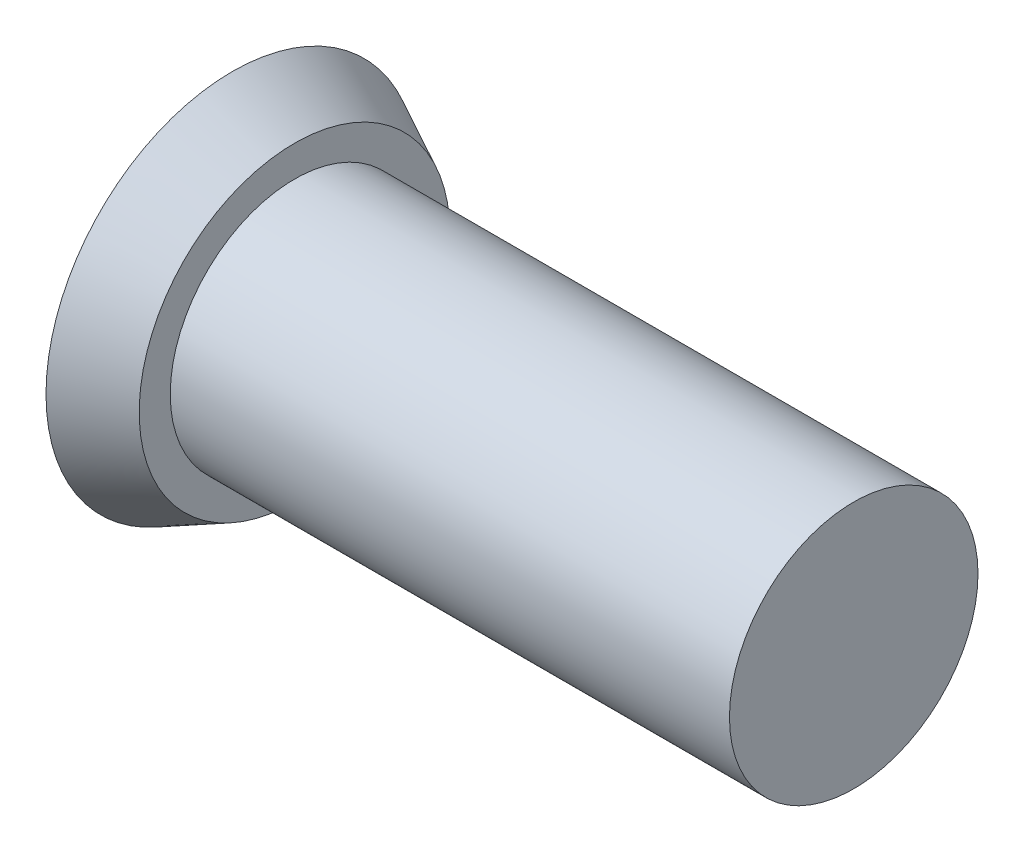
SolidWorks part; units mm, degrees
ref_plane "Front Plane" through (0, 0, 0) normal (0, 0, 1) x (1, 0, 0)
ref_plane "Top Plane" through (0, 0, 0) normal (0, 1, 0) x (1, 0, 0)
ref_plane "Right Plane" through (0, 0, 0) normal (1, 0, 0) x (0, 0, -1)
other "Configuration Table"
sketch "Sketch1" plane through (0, 0, 0) normal (0, 0, 1) x (1, 0, 0)
  line L0 (0, 0) -> (0, 3)
  line L1 (0, 3) -> (1, 2.5)
  line L2 (1, 2.5) -> (1, 2)
  line L3 (1, 2) -> (10, 2)
  line L4 (10, 2) -> (10, 0)
  line L5 (10, 0) -> (0, 0)
  dimension "D1" = 10
  dimension "D2" = 3
  dimension "D3" = 2.5
  dimension "D4" = 1
  dimension "D5" = 2
revolve "Revolve1" add sketch "Sketch1" angle 360 about L5
